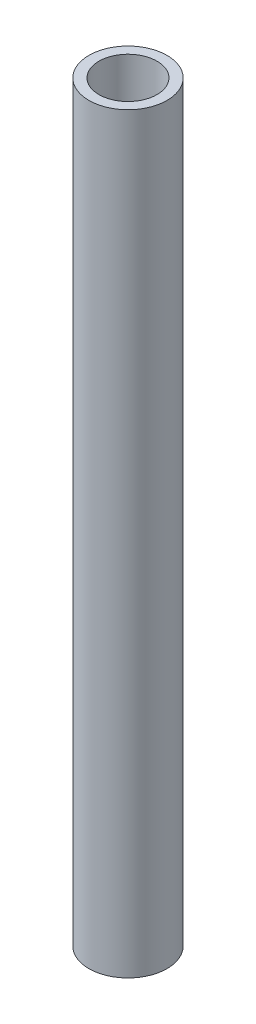
SolidWorks part; units mm, degrees
ref_plane "前基準面" through (0, 0, 0) normal (0, 0, 1) x (1, 0, 0)
ref_plane "上基準面" through (0, 0, 0) normal (0, 1, 0) x (1, 0, 0)
ref_plane "右基準面" through (0, 0, 0) normal (1, 0, 0) x (0, 0, -1)
sketch "草图1" plane through (0, 0, 0) normal (0, 1, 0) x (1, 0, 0)
  circle A0 centre (0, 0) radius 17.5
  dimension "D1" = 35
extrude "凸台-拉伸1" add sketch "草图1" along normal blind 337
shell "抽壳1" thickness 4.5
